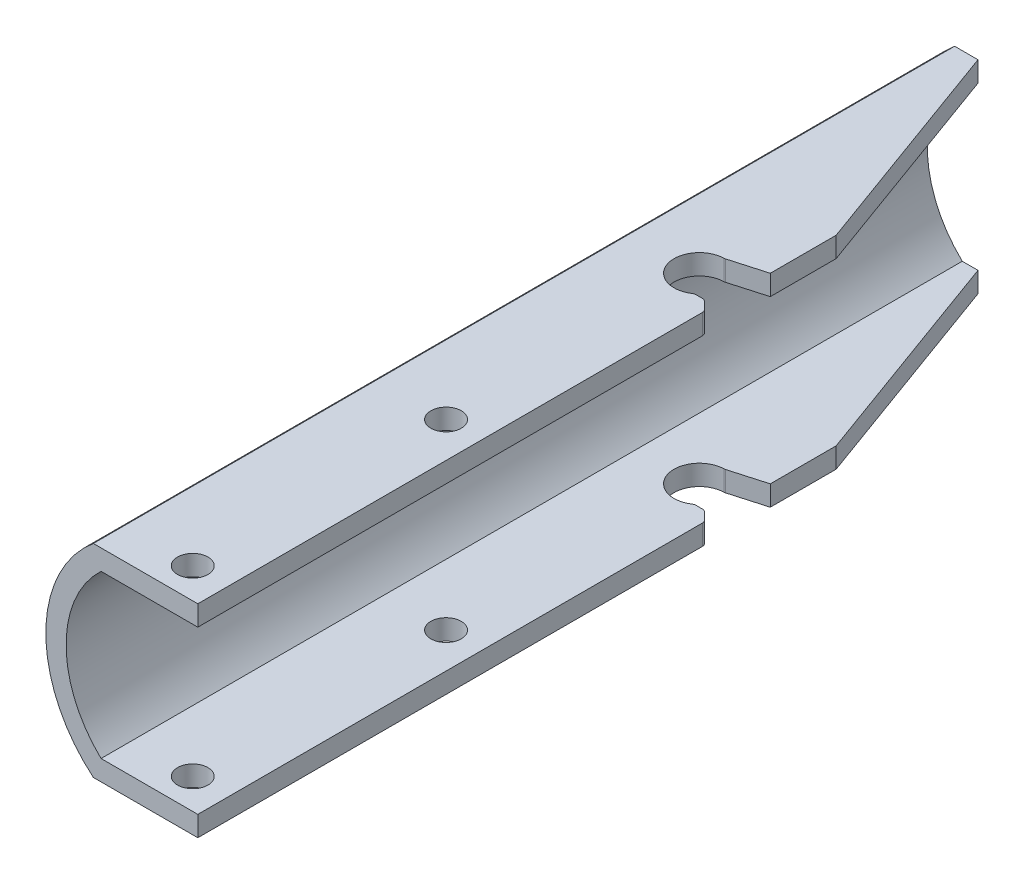
SolidWorks part; units mm, degrees
ref_plane "Front Plane" through (0, 0, 0) normal (0, 0, 1) x (1, 0, 0)
ref_plane "Top Plane" through (0, 0, 0) normal (0, 1, 0) x (1, 0, 0)
ref_plane "Right Plane" through (0, 0, 0) normal (1, 0, 0) x (0, 0, -1)
other "Configuration Table"
sketch "Sketch1" plane through (0, 0, 0) normal (0, 0, 1) x (1, 0, 0)
  line L0 (-8.3066, 10) -> (2, 10)
  line L2 (-7.5498, 8) -> (2, 8)
  line L3 (-7.5498, -8) -> (2, -8)
  line L6 (-8.3066, -10) -> (2, -10)
  line L7 (2, -8) -> (2, -10)
  line L8 (2, 8) -> (2, 10)
  arc A0 (-7.5498, 8) -> (-7.5498, -8) centre (0, 0) ccw
  arc A1 (-8.3066, 10) -> (-8.3066, -10) centre (0, 0) ccw
  dimension "D1" = 22
  dimension "D2" = 16
  dimension "D3" = 2
  dimension "D4" = 8
  dimension "D5" = 2
extrude "Boss-Extrude1" add sketch "Sketch1" along normal blind 85
sketch "Sketch2" plane through (0, -10, 0) normal (0, -1, 0) x (-1, 0, 0)
  line L0 (-2, -85) -> (-2, 0) construction
  line L1 (8.3066, -85) -> (-2, -85) construction
  line L2 (-2, -22) -> (6, 0)
  line L3 (8.3066, 0) -> (-2, 0) construction
  line L4 (6, 0) -> (-2, 0)
  line L5 (-2, 0) -> (-2, -22)
  circle A0 centre (1.5, -82) radius 1.5
  circle A1 centre (1.5, -57) radius 1.5
  dimension "D1" = 3
  dimension "D2" = 3.5
  dimension "D3" = 3
  dimension "D4" = 3
  dimension "D5" = 28
  dimension "D6" = 22
  dimension "D7" = 8
extrude "Cut-Extrude1" cut sketch "Sketch2" against normal through all
sketch "Sketch3" plane through (0, -10, 0) normal (0, -1, 0) x (-1, 0, 0)
  line L0 (1.5, -82) -> (1.5, -28.816) construction
  line L1 (-2, -28.5) -> (-2, -35)
  line L2 (0, -34) -> (-1, -34)
  line L3 (1.5, -29.5) -> (-2, -28.5)
  line L4 (-2, -85) -> (-2, -22) construction
  line L5 (-1, -34) -> (-2, -35)
  arc A0 (0, -34) -> (1.5, -29.5) centre (1.5, -32) ccw
  circle A1 centre (1.5, -82) radius 1.5 construction
  dimension "D1" = 50
  dimension "D2" = 2.5
  dimension "D3" = 2
  dimension "D4" = 3.5
  dimension "D5" = 45
  dimension "D6" = 1
extrude "Cut-Extrude2" cut sketch "Sketch3" against normal through all
fillet "Fillet1" radius 0.5 6 edges at (0, -9, 34) (0, 9, 34) (2, -9, 35) (1, -9, 34) (1, 9, 34) (2, 9, 35)
fillet "Fillet2" radius 0.5 2 edges at (-1.5, 9, 29.5) (-1.5, -9, 29.5)
